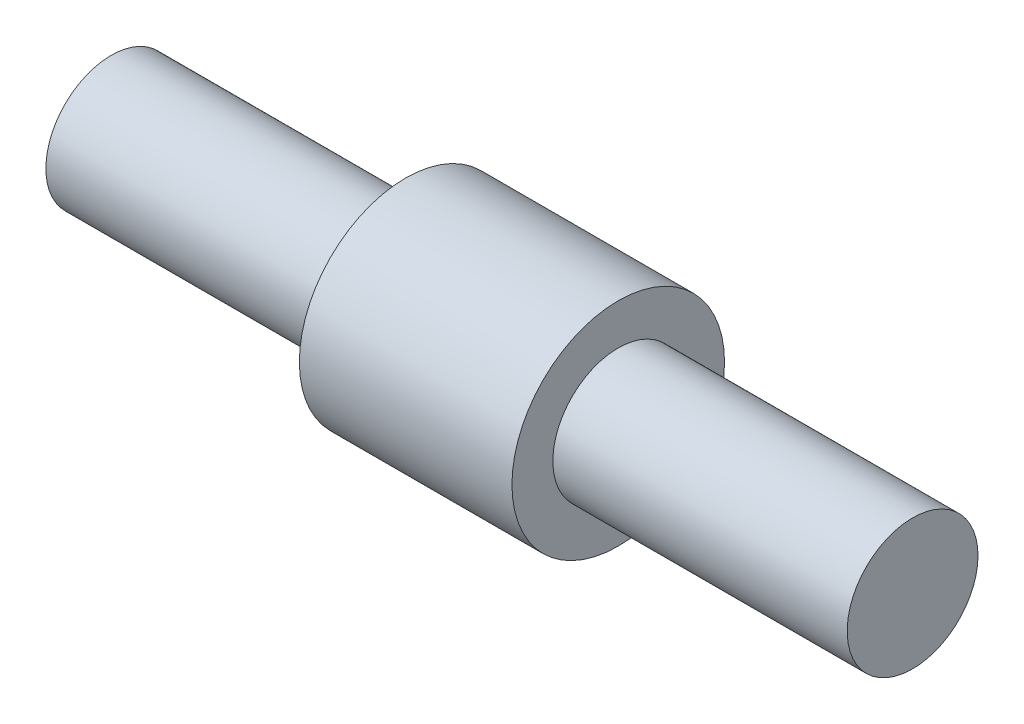
from build123d import *

# Parameters (mm, degrees)
SKETCH1_R           = 6.5
BOSS_EXTRUDE1_DEPTH = 6.5
SKETCH3_R           = 4
BOSS_EXTRUDE2_DEPTH = 18


with BuildPart() as part:
    # Sketch1 → Boss-Extrude1 (new, symmetric)
    with BuildSketch(Plane(origin=(0, 0, 0), x_dir=(0, 0, -1), z_dir=(1, 0, 0))):
        with Locations(Location((0, 0, 0), (0, 0, 180))):
            Circle(SKETCH1_R)
    extrude(amount=BOSS_EXTRUDE1_DEPTH, both=True)

    # Sketch3 → Boss-Extrude2 (add)
    with BuildSketch(Plane(origin=(6.5, 0, 0), x_dir=(0, 0, -1), z_dir=(1, 0, 0))):
        Circle(SKETCH3_R)
    boss_extrude2 = extrude(amount=BOSS_EXTRUDE2_DEPTH)

    # Mirror1: Boss-Extrude2 across plane
    add(boss_extrude2.mirror(Plane(origin=(0, 0, 0), x_dir=(0, 0, 1), z_dir=(1, 0, 0))))


solid = part.part
